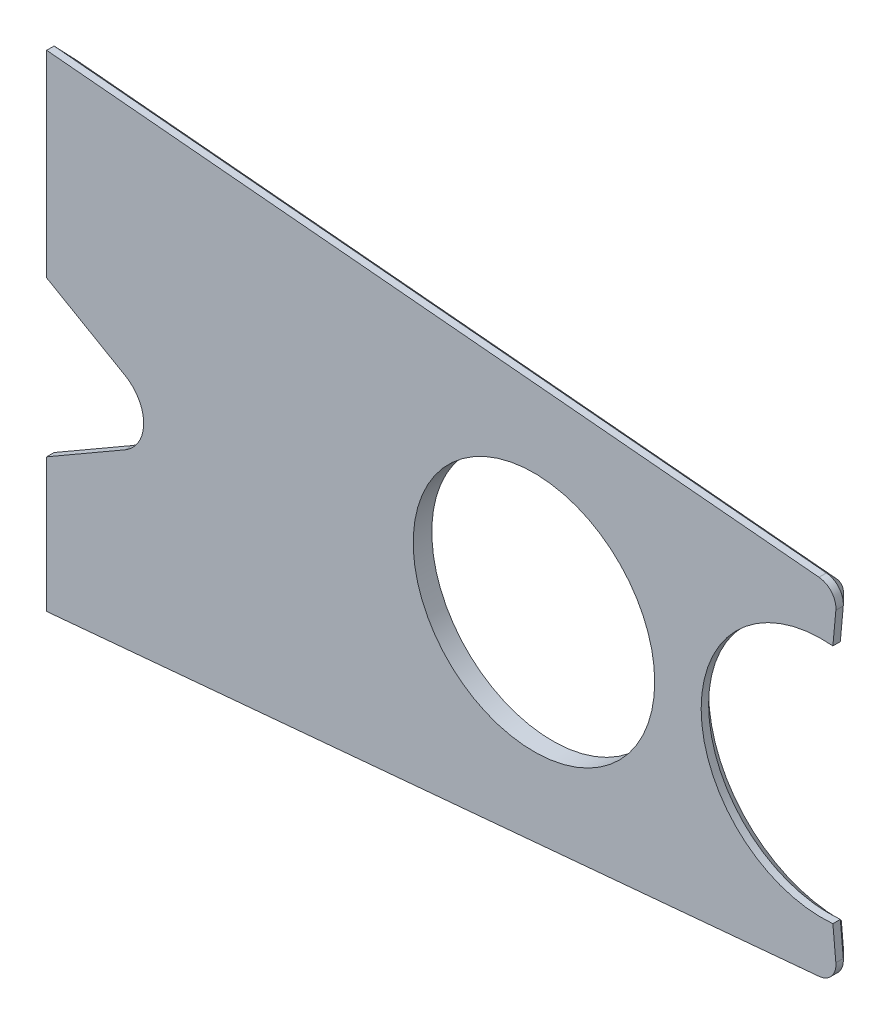
SolidWorks part; units mm, degrees
ref_plane "Front Plane" through (0, 0, 0) normal (0, 0, 1) x (1, 0, 0)
ref_plane "Top Plane" through (0, 0, 0) normal (0, 1, 0) x (1, 0, 0)
ref_plane "Right Plane" through (0, 0, 0) normal (1, 0, 0) x (0, 0, -1)
sketch "Sketch1" plane through (0, 0, 0) normal (0, 0, 1) x (1, 0, 0)
  line L0 (-94.5847, 0) -> (177.0221, 0) construction
  line L1 (155, 125.9672) -> (155, -105.1174) construction
  line L2 (-262.3, 130.8) -> (-262.3, 24.7)
  line L3 (-262.3, 130.8) -> (153.441, 93.0228)
  line L4 (-262.3, -130.8) -> (153.441, -93.0228)
  line L5 (162.4951, 82.1588) -> (160.9114, 64.7306)
  line L6 (162.4951, -82.1588) -> (160.9114, -64.7306)
  line L9 (-262.3, -58.7) -> (-220.0735, -34.3205)
  line L10 (-262.3, 24.7) -> (-220.0735, 0.3205)
  line L11 (-262.3, -58.7) -> (-262.3, -130.8)
  circle A0 centre (0, 0) radius 65
  arc A1 (160.9114, 64.7306) -> (160.9114, -64.7306) centre (155, 0) ccw
  arc A2 (-220.0735, 0.3205) -> (-220.0735, -34.3205) centre (-230.0735, -17) cw
  arc A3 (163.3707, -92.1205) -> (163.3707, 92.1205) centre (155, 0) ccw construction
  arc A4 (162.4951, 82.1588) -> (153.441, 93.0228) centre (152.5361, 83.0638) ccw
  arc A5 (162.4951, -82.1588) -> (153.441, -93.0228) centre (152.5361, -83.0638) cw
  point P24 (163.4, 92.1178)
  point P27 (163.4, -92.1178)
  dimension "D1" = 130
  dimension "D3" = 130
  dimension "D9" = 10
  dimension "D17" = 20
  dimension "D7" = 185
  dimension "D2" = 155
  dimension "D4" = 262.3
  dimension "D5" = 130.8
  dimension "D6" = 261.6
  dimension "D8" = 8.4
  dimension "D13" = 72.1
  dimension "D14" = 83.4
  dimension "D15" = 60
  dimension "D16" = 30
extrude "Boss-Extrude1" add sketch "Sketch1" along normal blind 10
chamfer "Chamfer1" distance 6 angle 45 12 edges at (-54.4295, 111.9114, 0) (-262.3, 77.75, 0) (-241.1867, 12.5103, 0) (-210.0735, -17, 0) (-241.1867, -46.5103, 0) (-262.3, -94.75, 0) (-54.4295, -111.9114, 0) (161.7032, -73.4447, 0) (90, 0, 0) (161.7032, 73.4447, 0) (160.218, 89.4659, 0) (160.218, -89.4659, 0)
